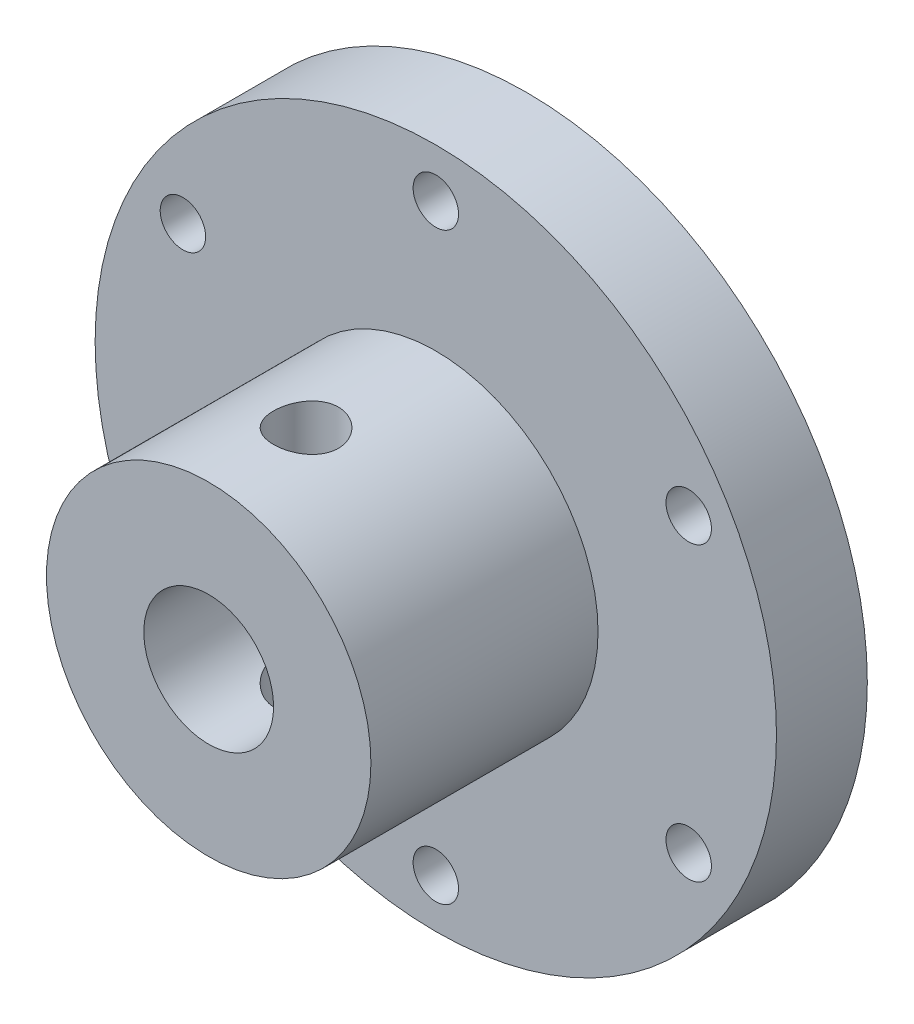
SolidWorks part; units mm, degrees
ref_plane "Front Plane" through (0, 0, 0) normal (0, 0, 1) x (1, 0, 0)
ref_plane "Top Plane" through (0, 0, 0) normal (0, 1, 0) x (1, 0, 0)
ref_plane "Right Plane" through (0, 0, 0) normal (1, 0, 0) x (0, 0, -1)
other "Configuration Table"
sketch "Sketch1" plane through (0, 0, 0) normal (0, 0, 1) x (1, 0, 0)
  circle A0 centre (0, 0) radius 52.5
  circle A1 centre (0, 0) radius 45 construction
  circle A2 centre (0, 45) radius 3.5
  circle A3 centre (38.9711, 22.5) radius 3.5
  circle A4 centre (38.9711, -22.5) radius 3.5
  circle A5 centre (0, -45) radius 3.5
  circle A6 centre (-38.9711, -22.5) radius 3.5
  circle A7 centre (-38.9711, 22.5) radius 3.5
  point P19 (0, 0)
  dimension "D1" = 105
  dimension "D2" = 90
  dimension "D3" = 7
  dimension "D4" = 6
extrude "Boss-Extrude1" add sketch "Sketch1" along normal blind 14
sketch "Sketch2" plane through (0, 0, 14) normal (0, 0, 1) x (1, 0, 0)
  circle A0 centre (0, 0) radius 25
  circle A1 centre (0, 0) radius 10
  dimension "D1" = 50
  dimension "D2" = 20
extrude "Boss-Extrude2" add sketch "Sketch2" along normal blind 35
sketch "Sketch3" plane through (0, 0, 0) normal (0, 1, 0) x (1, 0, 0)
  line L0 (-25, -14) -> (25, -14) construction
  circle A0 centre (0, -34) radius 5
  dimension "D1" = 10
  dimension "D2" = 20
extrude "Cut-Extrude1" cut sketch "Sketch3" against normal through all both and the other way through all
